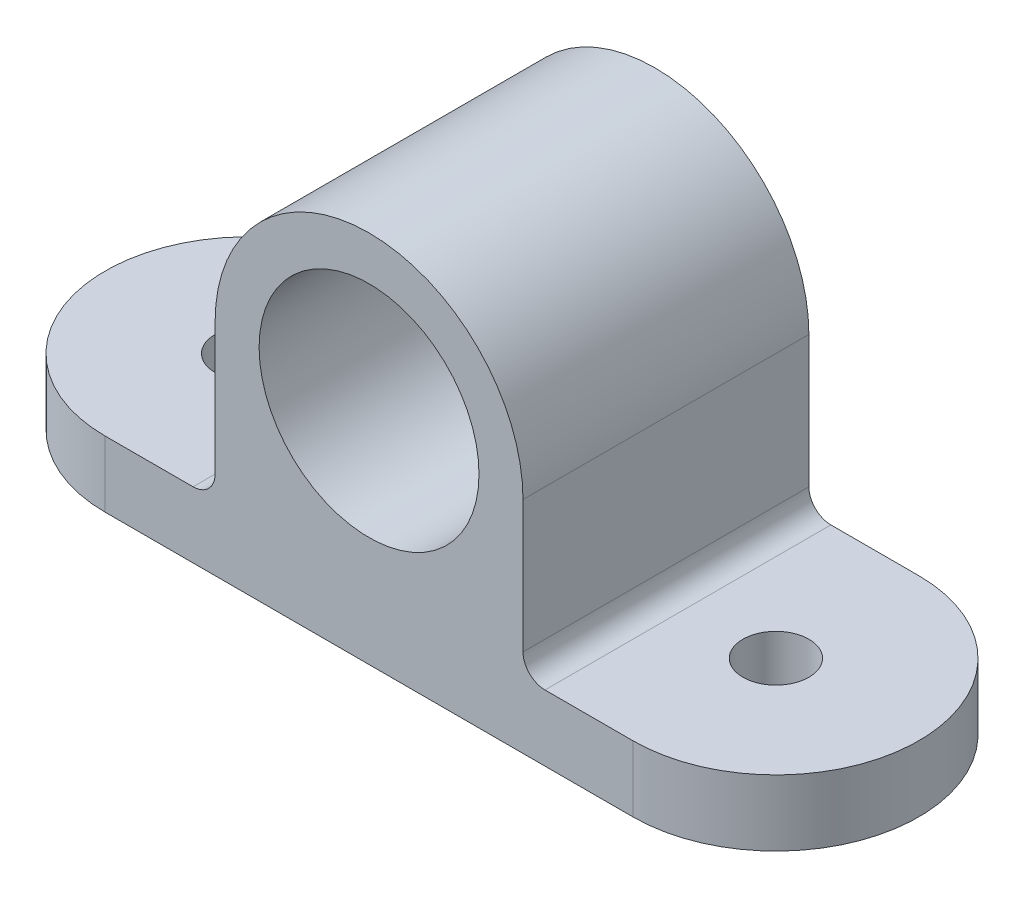
from build123d import *

# Parameters (mm, degrees)
SKETCH1_R           = 3
BOSS_EXTRUDE1_DEPTH = 6
SKETCH2_R           = 10
BOSS_EXTRUDE2_DEPTH = 13
FILLET1_R           = 2


with BuildPart() as part:
    # Sketch1 → Boss-Extrude1 (new body)
    with BuildSketch(Plane(origin=(0, 0, 0), x_dir=(1, 0, 0), z_dir=(0, 1, 0))):
        with BuildLine():
            Line((-24, 13), (24, 13))
            ThreePointArc((24, 13), (37, 0), (24, -13))
            Line((24, -13), (-24, -13))
            ThreePointArc((-24, -13), (-37, 0), (-24, 13))
        make_face()
        with Locations(Location((-24, 0, 0), (0, 0, 270))):
            Circle(SKETCH1_R, mode=Mode.SUBTRACT)
        with Locations(Location((24, 0, 0), (0, 0, 270))):
            Circle(SKETCH1_R, mode=Mode.SUBTRACT)
    extrude(amount=BOSS_EXTRUDE1_DEPTH)

    # Sketch2 → Boss-Extrude2 (add, symmetric)
    with BuildSketch(Plane.XY):
        with BuildLine():
            Line((-14, 20), (-14, 0))
            Line((-14, 0), (14, 0))
            Line((14, 0), (14, 20))
            ThreePointArc((14, 20), (0, 34), (-14, 20))
        make_face()
        with Locations(Location((0, 20, 0), (0, 0, 180))):
            Circle(SKETCH2_R, mode=Mode.SUBTRACT)
    extrude(amount=BOSS_EXTRUDE2_DEPTH, both=True)

    # Fillet1
    fillet1_edges = [part.edges().sort_by_distance(p)[0] for p in [
        (-14, 6, 0),
        (14, 6, 0),
    ]]
    fillet(fillet1_edges, radius=FILLET1_R)


solid = part.part
